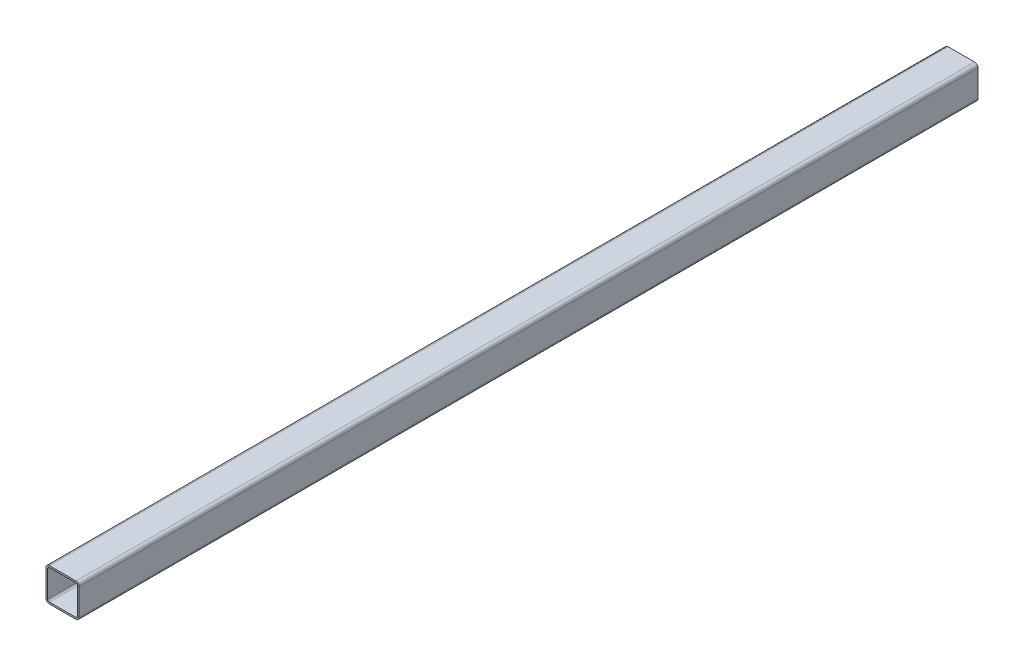
SolidWorks part; units mm, degrees
material "Q235A"
ref_plane "Front Plane" through (0, 0, 0) normal (0, 0, 1) x (1, 0, 0)
ref_plane "Top Plane" through (0, 0, 0) normal (0, 1, 0) x (1, 0, 0)
ref_plane "Right Plane" through (0, 0, 0) normal (1, 0, 0) x (0, 0, -1)
sketch "Sketch1" plane through (0, 0, 0) normal (0, 0, 1) x (1, 0, 0)
  line L1 (-20, 20) -> (20, 20)
  line L2 (-20, 20) -> (-20, -20)
  line L3 (-20, -20) -> (20, -20)
  line L4 (20, 20) -> (20, -20)
  line L5 (-20, 20) -> (20, -20) construction
  line L6 (-20, -20) -> (20, 20) construction
  line L7 (-18, 18) -> (18, 18)
  line L8 (-18, 18) -> (-18, -18)
  line L9 (-18, -18) -> (18, -18)
  line L10 (18, 18) -> (18, -18)
  line L11 (-18, 18) -> (18, -18) construction
  line L12 (-18, -18) -> (18, 18) construction
  point P0 (0, 0)
  point P6 (0, 0)
  dimension "D1" = 40
  dimension "D2" = 40
  dimension "D3" = 2
  dimension "D4" = 2
extrude "Boss-Extrude1" add sketch "Sketch1" along normal blind 1082
fillet "Fillet1" radius 2 4 edges at (18, 18, 541) (-18, 18, 541) (-18, -18, 541) (18, -18, 541)
fillet "Fillet2" radius 4 4 edges at (20, 20, 541) (20, -20, 541) (-20, 20, 541) (-20, -20, 541)
